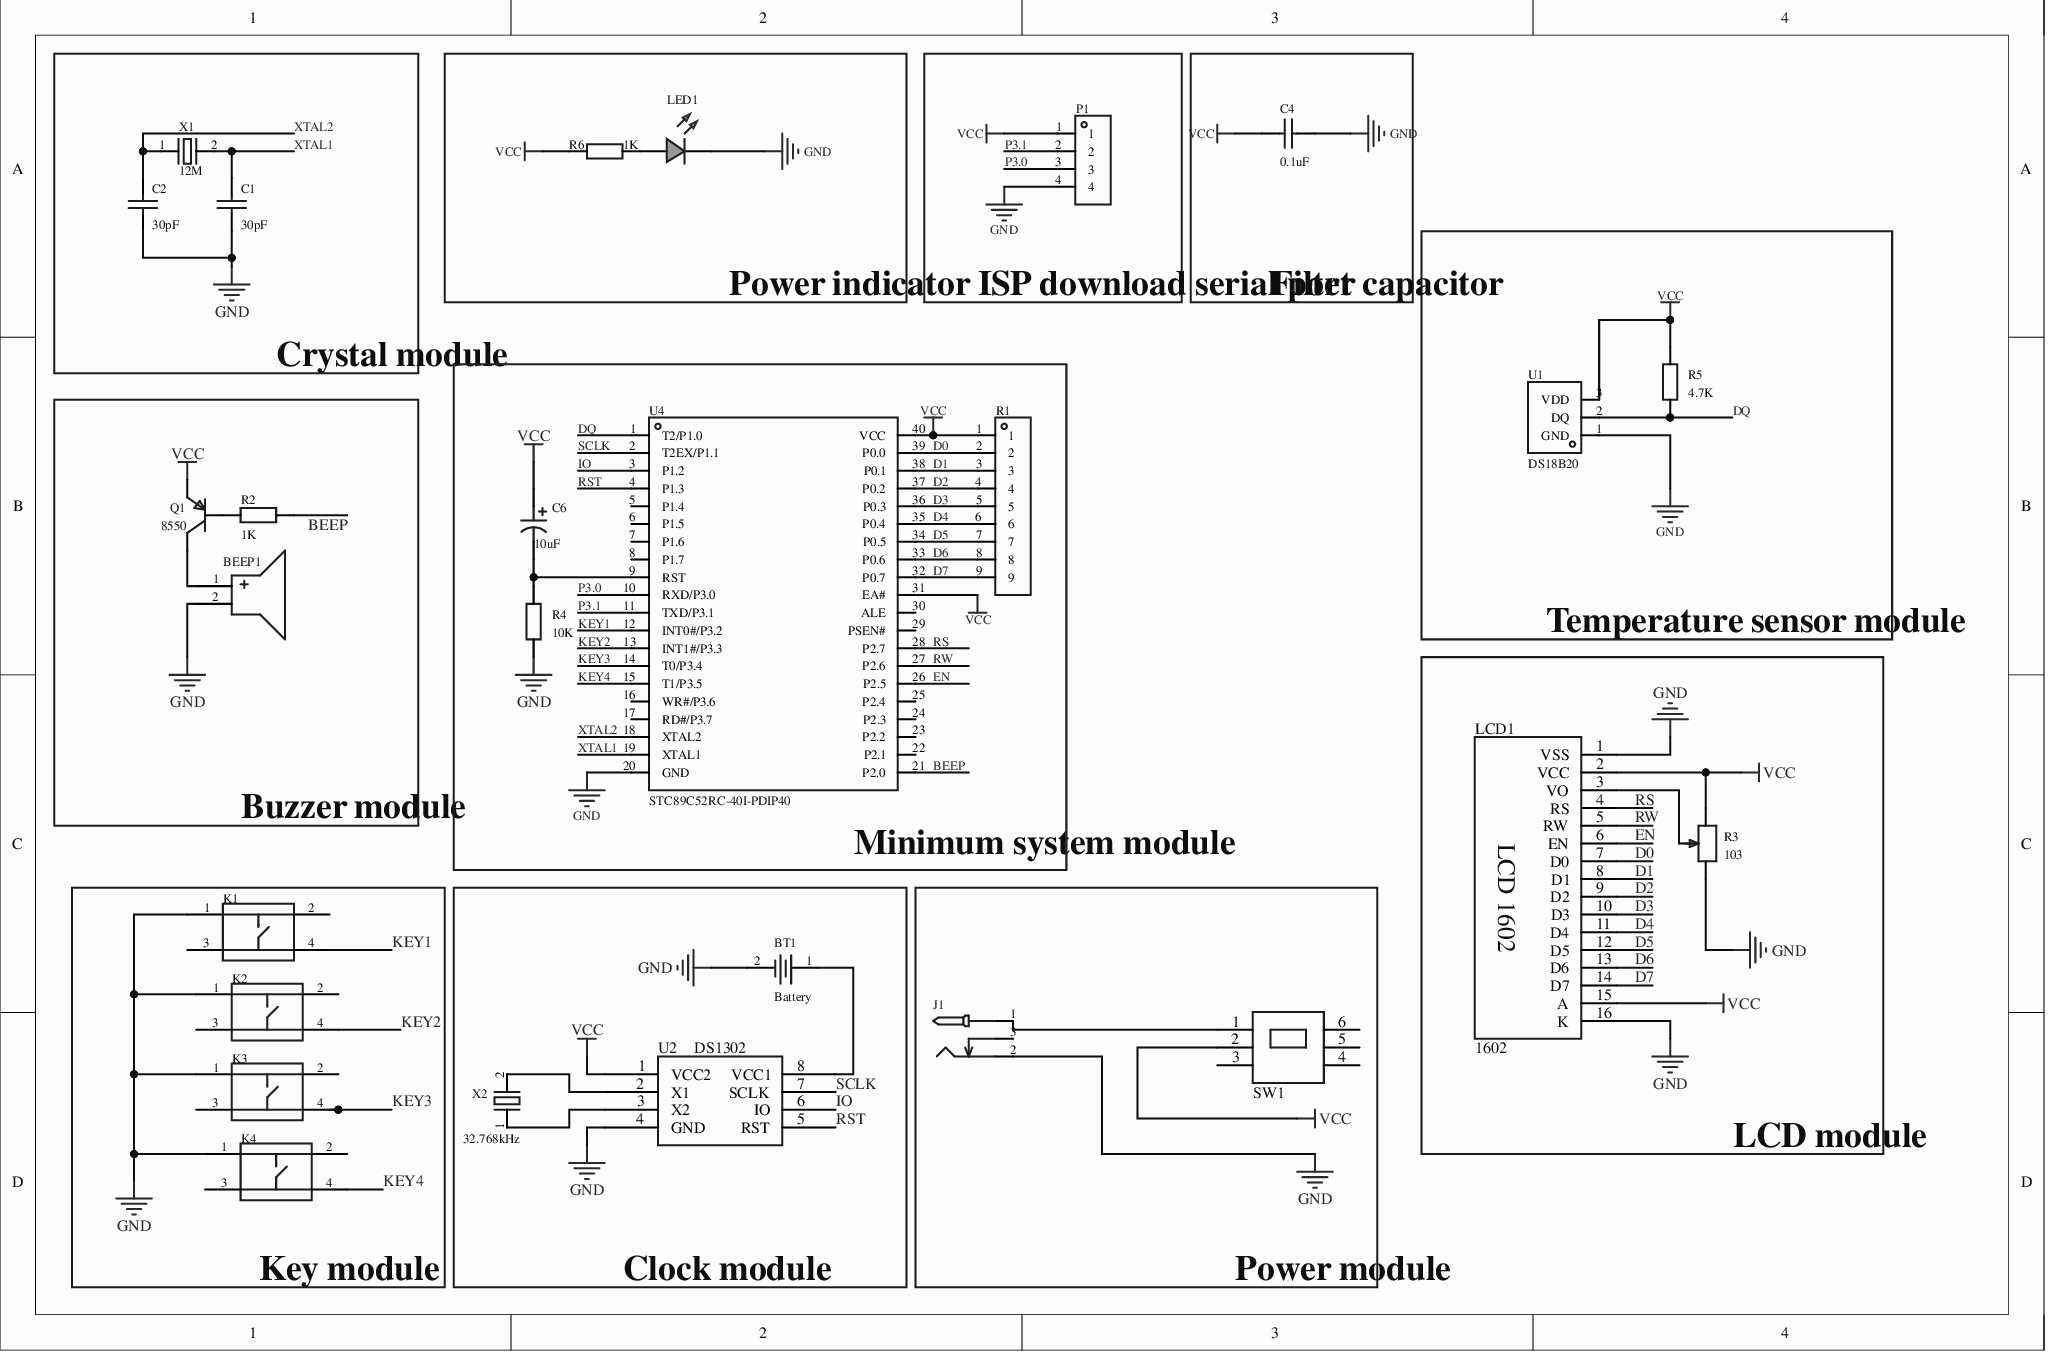
[diagram p0: MISC51325-2.schdoc]
# Altium project MISC51325-3.PrjPcb
1 sheet, 27 parts. Net scope: global (net labels, ports and power ports of the same name join across sheets).
Board file: MISC51325.pcbdoc

## Sheet MISC51325-2.schdoc
size 292 x 193 mm; Name: MISC51325

### Parts
BEEP1  (no value)  [BUZ-TH_BD12.0-P7.60-D0.6-FD]
BT1  Battery  [BAT-TH_CR2032]
C1  30pF  [CAP-TH_L5.0-W4.0-P5.00-D1.0]
C2  30pF  [CAP-TH_L5.0-W4.0-P5.00-D1.0]
C4  0.1uF  [CAP-TH_L5.0-W4.0-P5.00-D1.0]
C6  10uF  [CAP-TH_BD5.0-P2.00-D0.6-FD]
J1  (no value)  [DC-005_2.5]
K1  (no value)  [KEY-TH_4P-L6.0-W6.0-P4.50-LS6.50]
K2  (no value)  [KEY-TH_4P-L6.0-W6.0-P4.50-LS6.50]
K3  (no value)  [KEY-TH_4P-L6.0-W6.0-P4.50-LS6.50]
K4  (no value)  [KEY-TH_4P-L6.0-W6.0-P4.50-LS6.50]
LCD1  1602  [HDR-M-2.54_1X16]
LED1  (no value)  [LED-TH_5mm]
P1  (no value)  [HDR-TH_4P-P2.54-V-M]
Q1  8550  [S8550P_TO-92]
R1  (no value)  [SIP-9_L22.3-W3.2-P2.54_KA2284-SIP-9]
R2  1K  [Res_1/4W]
R3  103  [RES-ADJ-SMD_RM065-V1]
R4  10K  [Res_1/4W]
R5  4.7K  [Res_1/4W]
R6  1K  [Res_1/4W]
SW1  SWT  [SW-TH_6P-L8.5-W8.5-P2.50-LS5.5-BL-2]  (value not drawn)
U1  DS18B20  [TO-92-3_L4.5-W3.5-P1.27-L]
U2  DS1302  [DIP-8_L10.9-W6.4-P2.54-LS7.6-BL]
U4  STC89C52RC-40I-PDIP40  [DIP-40_L52.0-W13.7-P2.54-LS15.2-BL]
X1  12M  [HC-49S_L11.5-W4.7-P4.88]
X2  32.768kHz  [CRYSTAL-TH_BD1.4-P0.45-D0.2]

### Blocks framed on the sheet
Crystal module: C1 C2 X1
Power indicator: LED1 R6
ISP download serial port: P1
Filter capacitor: C4
Temperature sensor module: R5 U1
Minimum system module: C6 R1 R4 U4
Buzzer module: BEEP1 Q1 R2
LCD module: LCD1 R3
Key module: K1-K4
Clock module: BT1 U2 X2
Power module: J1 SW1

### Nets
GND: BEEP1.2(-) BT1.2 C1.1 C2.1 C4.2 J1.2 K1.1 K2.1 K3.1 K4.1 LCD1.1(VSS) LCD1.16(K) LED1.2(A) P1.4 R3.1 R4.1 U1.1(GND) U2.4(GND) U4.20(GND)
VCC: C4.1 C6.1 LCD1.2(VCC) LCD1.15(A) P1.1 Q1.1(E) R1.1 R3.3 R5.2 R6.1 SW1.2 U1.3(VDD) U2.1(VCC2) U4.31(EA#) U4.40(VCC)
BEEP: R2.2 U4.21(P2.0)
D0: LCD1.7(D0) R1.2 U4.39(P0.0)
D1: LCD1.8(D1) R1.3 U4.38(P0.1)
D2: LCD1.9(D2) R1.4 U4.37(P0.2)
D3: LCD1.10(D3) R1.5 U4.36(P0.3)
D4: LCD1.11(D4) R1.6 U4.35(P0.4)
D5: LCD1.12(D5) R1.7 U4.34(P0.5)
D6: LCD1.13(D6) R1.8 U4.33(P0.6)
D7: LCD1.14(D7) R1.9 U4.32(P0.7)
DQ: R5.1 U1.2(DQ) U4.1(T2/P1.0)
EN: LCD1.6(EN) U4.26(P2.5)
IO: U2.6(IO) U4.3(P1.2)
KEY1: K1.4 U4.12(INT0#/P3.2)
KEY2: K2.4 U4.13(INT1#/P3.3)
KEY3: K3.4 U4.14(T0/P3.4)
KEY4: K4.4 U4.15(T1/P3.5)
P3.0: P1.3 U4.10(RXD/P3.0)
P3.1: P1.2 U4.11(TXD/P3.1)
RS: LCD1.4(RS) U4.28(P2.7)
RST: U2.5(RST) U4.4(P1.3)
RW: LCD1.5(RW) U4.27(P2.6)
SCLK: U2.7(SCLK) U4.2(T2EX/P1.1)
XTAL1: C1.2 U4.19(XTAL1) X1.2
XTAL2: C2.2 U4.18(XTAL2) X1.1
NetBEEP1_1: BEEP1.1(+) Q1.3(C)
NetBT1_1: BT1.1 U2.8(VCC1)
NetC6_2: C6.2 R4.2 U4.9(RST)
NetJ1_1: J1.1 SW1.1
NetLCD1_3: LCD1.3(VO) R3.2
NetLED1_1: LED1.1(C) R6.2
NetQ1_2: Q1.2(B) R2.1
NetU2_2: U2.2(X1) X2.2
NetU2_3: U2.3(X2) X2.1

Not connected (* = marked no-connect by the designer): J1 3*; K1 2* 3*; K2 2* 3*; K3 2* 3*; K4 2* 3*; SW1 3(2)* 4(3)* 5(4)* 6(5)*; U4 5(P1.4)* 6(P1.5)* 7(P1.6)* 8(P1.7)* 16(WR#/P3.6)* 17(RD#/P3.7)* 22(P2.1)* 23(P2.2)* 24(P2.3)* 25(P2.4)* 29(PSEN#)* 30(ALE)*

### Library data of the parts
BEEP1 = BZ-D12-L7_6: AddInBom: yes; ModelId: 16ab50e14c5b4f2c986c135bdba60e370819f05c4eef4c71ace90d822a990e87; ModelName: BUZ-TH_D12.0-H9.5-P7.60; ModelTransform: 472.44,472.176,0,90,0,0,-0.787,0,-177.165; Symbol: BZ-D12-L7_6; Device: BZ-D12-L7_6; LCSC Part Name: BZ-D12-L7_6; SupplierPart: C9900009978; Supplier Footprint: BUZ-TH; JLCPCB Part Class: Extended Part; Supplier: LCSC; ConvertToPcb: yes; FootprintName: BUZ-TH_BD12.0-P7.60-D0.6-FD
BT1 = Q&J CR2032 20-6*9_C9900112302: AddInBom: yes; ModelId: 2a22c62c6e424c70bca0a6138eddf4b70819f05c4eef4c71ace90d822a990e87; ModelTransform: 814.959,786.69055,0,180,0,0,0,0,-196.85; Symbol: Q&J CR2032 20-6*9; Device: Q&J CR2032 20-6*9_C9900112302; Manufacturer Part: Battery; LCSC Part Name: Q&J CR2032 20-6*9; SupplierPart: C9900112302; Supplier Footprint: BAT-TH_CR2032; JLCPCB Part Class: Extended Part; Supplier: LCSC; ConvertToPcb: yes; FootprintName: BAT-TH_CR2032; ModelName: BAT-TH_CR2032
C1 C2 C4 = 瓷片电容47PF 3KV: Capacitance: -; rated voltage: -; temperature coefficient: -;; Symbol: Ceramic capacitors47PF 3KV; Device: Ceramic capacitor 47PF 3KV; AddInBom: yes; ModelId: 7562e8dfad8b481384451709c5473ca60819f05c4eef4c71ace90d822a990e87; ModelName: CAP-TH_BD5.0-W4.0-P5.08; ModelTransform: 224.49711,157.48,0,0,0,0,0,0,-137.795; LCSC Part Name: 47pF(47R) ±10% 3KV; ManufacturerPart: 瓷片电容47PF 3KV; Supplier Footprint: 插件; JLCPCB Part Class: Extended Part; Supplier: LCSC; ConvertToPcb: yes; FootprintName: CAP-TH_L5.0-W4.0-P5.00-D1.0; Voltage Rated: -; Lead Spacing: -; Temperature Coefficient: -; φD: -; Body Thickness: -
  C1 C2: Value: 30pF
  C4: Value: 0.1uF
C6 = 10uF/25V-C5X11DIP: AddInBom: yes; ModelId: e14933aa819f4e768454ffe1b66cd5400819f05c4eef4c71ace90d822a990e87; ModelTransform: 196.70055,196.77528,0,0,0,0,0.118,0,-137.795; Symbol: 10UF/25V-C5X11DIP; Device: 10uF/25V-C5X11DIP; Manufacturer Part: 10uF; LCSC Part Name: 10uF/25V-C5X11DIP; SupplierPart: C9900003841; Supplier Footprint: CAP-TH_BD5.0-P2.00; JLCPCB Part Class: Extended Part; Supplier: LCSC; ConvertToPcb: yes; FootprintName: CAP-TH_BD5.0-P2.00-D0.6-FD; ModelName: CAP-TH_BD5.0-P2.00-D0.6-FD
J1 = DC-005_2.5: ConvertToPcb: yes; ModelId: f168fe383f964e0ea2af0127ff6ac7b40819f05c4eef4c71ace90d822a990e87; ModelName: DC-IN-TH_DC005; ModelTransform: 366.14,553.15,590.55,90,0,0,137.8,-11.81,-157.48; Symbol: DC-005_2.5; Device: DC-005_2.5; AddInBom: yes; Supplier Footprint: 插件; FootprintName: DC-005_2.5
K1-K4 = K2-1102DP-C4SW-04: Circuit structure: SPST; button shape: round button; actuating force: 2.5N; mounting: through-hole; switch length: 6mm; switch width: 6mm; switch height: 5mm; contact current: 50mA; rated voltage: 12V; with light: -; operating life: 10 ten-thousand cycles;; Manufacturer: 韩国韩荣; AddInBom: yes; ModelId: b38fea4b2e4e408486f1d54ff7bc5cc00819f05c4eef4c71ace90d822a990e87; ModelTransform: 307.086,236.22,0,0,0,0,0,0,-137.795; Symbol: K2-1102DP-C4SW-04; Device: K2-1102DP-C4SW-04; LCSC Part Name: 轻触按键开关6*6*5; SupplierPart: C110153; Supplier Footprint: 插件-4P,6x6mm; JLCPCB Part Class: Extended Part; Datasheet: https://item.szlcsc.com/datasheet/K2-1102DP-C4SW-04/111374.html; Supplier: LCSC; ConvertToPcb: yes; FootprintName: KEY-TH_4P-L6.0-W6.0-P4.50-LS6.50; ModelName: KEY-TH_4P-L6.0-W6.0-P4.50-LS6.50; Circuit: SPST; Actuator Style: Round button; Operating Force: 2.5N; Mounting Type: Through-hole; Length: 6mm; Width: 6mm; Switch Height: 5mm; Contact Current: 50mA; Voltage Rating: 12V; With Lamp: -; Life: 10 ten-thousand cycles; Operating Temperature: -25℃~+85℃
LCD1 = 1602_1: AddInBom: yes; Device: 1602_1; DesignItemID: 1602; LibraryName: MANUAL; Symbol: 1602; FootprintName: HDR-M-2.54_1X16
LED1 = LED_TH-G_5mm: ConvertToPcb: yes; ModelId: fe7796f666a04da4b4289311169b45200819f05c4eef4c71ace90d822a990e87; ModelName: LED-TH_BD5.8-P2.54-FD_GREEN-1; ModelTransform: 212.58,227.91,537.36,0,0,0,-7.87,0,-196.85; Symbol: LED_TH-G; Device: LED_TH-G_5mm; AddInBom: yes; Supplier Footprint: 插件; FootprintName: LED-TH_5mm
P1 = HDR-M_2.54_1x4P: Symbol: PZ254V-11-04P; ConvertToPcb: yes; ModelId: 112f4d05e8d64e99ab9a333894bea4f90819f05c4eef4c71ace90d822a990e87; ModelName: HDR-TH_4P-P2.54-M-LI-1X4P; ModelTransform: 399.999,104.7242,0,0,0,0,0,0,-118.11; Device: HDR-M_2.54_1x4P; AddInBom: yes; SupplierPart: C492403; Supplier Footprint: 插件; FootprintName: HDR-TH_4P-P2.54-V-M
Q1 = S8550_TO_PNP: ConvertToPcb: yes; ModelId: aafe8e06f2154e7c93506efd0d6632dd0819f05c4eef4c71ace90d822a990e87; ModelName: TO-92-3_L4.9-W3.7-P1.27-L; ModelTransform: 180.78,141.44,417.3,0,0,0,0,0,-200; Symbol: S8550_TO_PNP; Device: S8550_TO_PNP; AddInBom: yes; Supplier Footprint: TO-92; FootprintName: S8550P_TO-92
R1 = HDR-M_2.54-1x9P: Symbol: PZ254V-11-09P; 3D Model: b5c1e988b3bb4503807579736b357ad00819f05c4eef4c71ace90d822a990e87; 3D Model Transform: 890.15562,98.425,0,0,0,0,0,0,-118.11; ConvertToPcb: yes; ModelName: HDR-TH_9P-P2.54-M-LI-1X9P; Device: HDR-M_2.54-1x9P; Supplier Part: C492408; Supplier Footprint: 插件; AddInBom: yes; FootprintName: SIP-9_L22.3-W3.2-P2.54_KA2284-SIP-9
R2 R4-R6 = Res_AXIAL-1/4W: Symbol: Resistor; 3D Model: 463263665006444ab7a47bd11b0cf9560819f05c4eef4c71ace90d822a990e87; 3D Model Transform: 427.165,94.32816,0,0,0,0,0,0,-196.85; AddInBom: yes; ModelName: RES-TH_BD2.4-L6.3-P10.30-D0.6; Device: Res_AXIAL-1/4W; Supplier Footprint: 轴向引线; ConvertToPcb: yes; FootprintName: Res_1/4W
  R2 R6: Value: 1K
  R4: Value: 10K
  R5: Value: 4.7K
R3 = RM065-V1-103: AddInBom: yes; ModelId: c816c2b7942147f5a832150e8ef6960c0819f05c4eef4c71ace90d822a990e87; ModelTransform: 255.905,283.464,0,0,0,0,0.025,-3.937,-157.48; Symbol: RM065-V1-103; Device: RM065-V1-103; Manufacturer Part: 103; LCSC Part Name: RM065-V1-103; SupplierPart: C54661; Supplier Footprint: -; JLCPCB Part Class: Extended Part; Supplier: LCSC; ConvertToPcb: yes; FootprintName: RES-ADJ-SMD_RM065-V1; ModelName: RES-ADJ-SMD_RM065-V1
SW1 = SWT_1: AddInBom: yes; Device: SWT_1; DesignItemID: SWT; LibraryName: Schlib; Symbol: SWT; FootprintName: SW-TH_6P-L8.5-W8.5-P2.50-LS5.5-BL-2
U1 = DS18B20: Detection temperature: -55℃~+125℃; accuracy: ±0.4℃; interface type: single-bus;; Manufacturer: HXY MOSFET(华轩阳电子); Symbol: DS18B20_C5451632; AddInBom: yes; ModelId: 45fa6cddef3743c6aacf8db740a3bc4c0819f05c4eef4c71ace90d822a990e87; ModelTransform: 177.165,137.795,0,0,0,0,0,29.528,-98.425; Voltage - Supply: 2.5V~5.5V; Standby Current: 1uA; Temperature Conversion Time: 400ms; Temperature Resolution: 12bit; Device: DS18B20; LCSC Part Name: 温度-10℃~70℃ 精度±0.4℃ 电压2.5V~5.5V; SupplierPart: C5451632; ManufacturerPart: DS18B20; Supplier Footprint: TO-92; JLCPCB Part Class: Extended Part; Datasheet: https://item.szlcsc.com/datasheet/DS18B20/6355375.html; Supplier: LCSC; ConvertToPcb: yes; FootprintName: TO-92-3_L4.5-W3.5-P1.27-L; ModelName: TO-92-3_L4.5-W3.5-P1.27-L; Detection Temperature Range: -55℃~+125℃; Tolerance: ±0.4℃; Interface: Single-bus; Operating Temperature: -
U2 = DS1302: AddInBom: yes; Device: DS1302; DesignItemID: DS1302; LibraryName: MANUAL; Symbol: DS1302; FootprintName: DIP-8_L10.9-W6.4-P2.54-LS7.6-BL
U4 = STC89C52RC-40I-PDIP40: CPU core: 51 family; maximum CPU frequency: -;; Manufacturer: STC; AddInBom: yes; ModelId: 16d4686a009b4ddca948f91eddb57b140819f05c4eef4c71ace90d822a990e87; ModelName: DIP-40_L52.3-W13.8-H4.0-LS15.24-P2.54; ModelTransform: 2059.051,615.743,0,0,0,0,0,0,-118.11; Program Storage Size: 8KB; Program Memory Type: FLASH; Voltage - Supply: 3.3V~5.5V; Symbol: STC89C52RC-40I; Device: STC89C52RC-40I-PDIP40; LCSC Part Name: 单片机原理及应用; SupplierPart: C14022; ManufacturerPart: STC89C52RC-40I-PDIP40; Supplier Footprint: DIP-40; JLCPCB Part Class: Extended Part; Datasheet: https://item.szlcsc.com/datasheet/STC89C52RC-40I-PDIP40/14679.html; Supplier: LCSC; ConvertToPcb: yes; FootprintName: DIP-40_L52.0-W13.7-P2.54-LS15.2-BL; CPU Core: 51 family; CPU Maximum Speed: -; RAM Size: -; EEPROM: -; Number of I/O: -; ADC (Bit): -; DAC (Bit): -
X1 = SWXSBBCVE0-16.000000: Crystal type: through-hole crystal; frequency: 16MHz; frequency tolerance at room temperature: ±20ppm; load capacitance: 12pF; frequency stability: ±30ppm;; Manufacturer: Starwave(思大); AddInBom: yes; ModelId: 8681f9edbc4c49baa7439b9863851e5c0819f05c4eef4c71ace90d822a990e87; ModelTransform: 452.755,183.4642,0,0,0,0,0,0,-137.795; Equivalent Series Resistance(ESR): 50Ω; Symbol: SWXSBBCVE0-16.000000; Device: SWXSBBCVE0-16.000000; Value: 12M; LCSC Part Name: 无源晶振; ManufacturerPart: SWXSBBCVE0-16.000000; Supplier Footprint: HC-49S; JLCPCB Part Class: Extended Part; Datasheet: https://item.szlcsc.com/datasheet/SWXSBBCVE0-16.000000/24100442.html; Supplier: LCSC; ConvertToPcb: yes; FootprintName: HC-49S_L11.5-W4.7-P4.88; ModelName: HC-49S_L11.5-W4.7-P4.88; Type: Through-hole crystal; Normal temperature Frequency Tolerance: ±20ppm; Load Capacitance: 12pF; Frequency Stability: ±30ppm; Operating Temperature: -40℃~+85℃
X2 = AB15T-32.768KHZ: Frequency: 32.768kHz; frequency tolerance at room temperature: ±20ppm; external load capacitance: 12.5pF; frequency stability (full temperature): -;; Manufacturer: ABRACON; AddInBom: yes; ModelId: 9fdeeb9d7ef84072bac6c58c302789500819f05c4eef4c71ace90d822a990e87; ModelTransform: 55.00706,55.09,0,0,0,0,0,0,-169.291; Equivalent Series Resistance (ESR): 40kΩ; Symbol: AB15T-32.768KHZ; Device: AB15T-32.768KHZ; LCSC Part Name: 32.768kHz ±20ppm 12.5pF; SupplierPart: C1669866; ManufacturerPart: AB15T-32.768KHZ; Supplier Footprint: DT-15; JLCPCB Part Class: Extended Part; Datasheet: https://atta.szlcsc.com/upload/public/pdf/source/20210504/0EA8EED362197519A7C3815AD65C577B.pdf; Supplier: LCSC; ConvertToPcb: yes; FootprintName: CRYSTAL-TH_BD1.4-P0.45-D0.2; ModelName: CRYSTAL-TH_BD1.4-P0.45-D0.2; Value: 32.768kHz; Normal temperature Frequency Tolerance: ±20ppm; External load capacitor: 12.5pF; Frequency Stability(Full temperature range): -; Operating Temperature: -20℃~+70℃